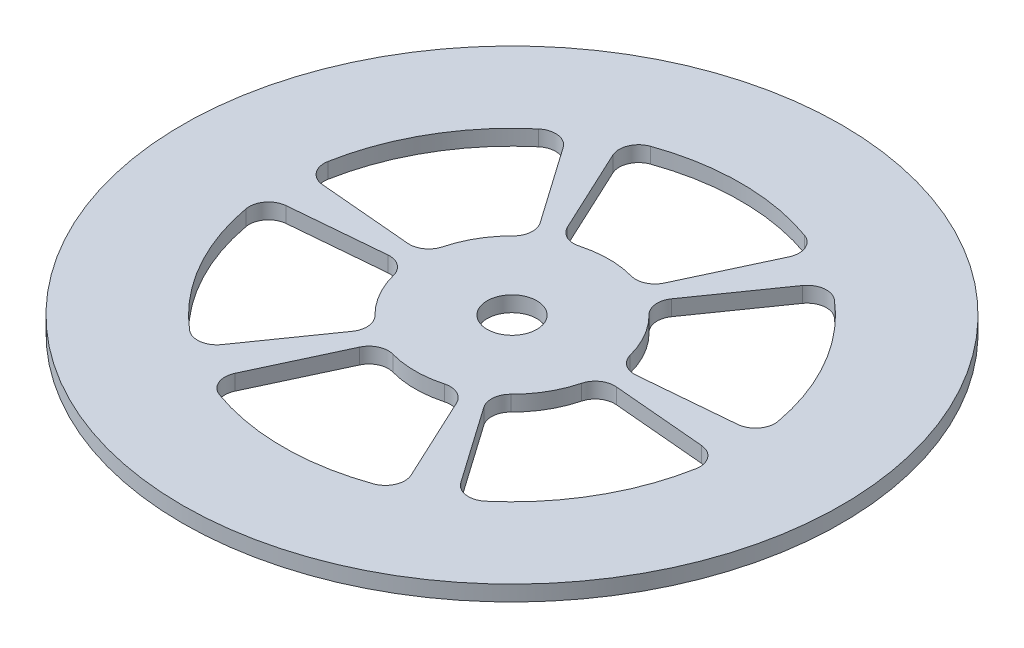
from build123d import *

# Parameters (mm, degrees)
SKETCH1_R           = 85
SKETCH1_R_2         = 6.4
BOSS_EXTRUDE1_DEPTH = 4
CUT_EXTRUDE1_DEPTH  = 10
FILLET1_R           = 5


with BuildPart() as part:
    # Sketch1 → Boss-Extrude1 (new body)
    with BuildSketch(Plane(origin=(0, 0, 0), x_dir=(1, 0, 0), z_dir=(0, 1, 0))):
        with Locations(Location((0, 0, 0), (0, 0, 270))):
            Circle(SKETCH1_R)
        with Locations(Location((0, 0, 0), (0, 0, 270))):
            Circle(SKETCH1_R_2, mode=Mode.SUBTRACT)
    extrude(amount=BOSS_EXTRUDE1_DEPTH)

    # Sketch2 → Cut-Extrude1 (cut)
    with BuildSketch(Plane(origin=(0, 4, 0), x_dir=(1, 0, 0), z_dir=(0, 1, 0))):
        with BuildLine():
            Line((10.565456544, 22.657694676), (24.934477443, 53.472159435))
            ThreePointArc((24.934477443, 53.472159435), (0, 59), (-24.934477443, 53.472159435))
            Line((-24.934477443, 53.472159435), (-10.565456544, 22.657694676))
            ThreePointArc((-10.565456544, 22.657694676), (0, 25), (10.565456544, 22.657694676))
        make_face()
        with BuildLine():
            Line((14.339410909, 20.478801107), (33.841009745, 48.329970613))
            ThreePointArc((33.841009745, 48.329970613), (51.095498823, 29.5), (58.775487187, 5.142188822))
            Line((58.775487187, 5.142188822), (24.904867452, 2.178893569))
            ThreePointArc((24.904867452, 2.178893569), (21.650635095, 12.5), (14.339410909, 20.478801107))
        make_face()
        with BuildLine():
            Line((24.904867452, -2.178893569), (58.775487187, -5.142188822))
            ThreePointArc((58.775487187, -5.142188822), (51.095498823, -29.5), (33.841009745, -48.329970613))
            Line((33.841009745, -48.329970613), (14.339410909, -20.478801107))
            ThreePointArc((14.339410909, -20.478801107), (21.650635095, -12.5), (24.904867452, -2.178893569))
        make_face()
        with BuildLine():
            Line((10.565456544, -22.657694676), (24.934477443, -53.472159435))
            ThreePointArc((24.934477443, -53.472159435), (0, -59), (-24.934477443, -53.472159435))
            Line((-24.934477443, -53.472159435), (-10.565456544, -22.657694676))
            ThreePointArc((-10.565456544, -22.657694676), (0, -25), (10.565456544, -22.657694676))
        make_face()
        with BuildLine():
            Line((-14.339410909, -20.478801107), (-33.841009745, -48.329970613))
            ThreePointArc((-33.841009745, -48.329970613), (-51.095498823, -29.5), (-58.775487187, -5.142188822))
            Line((-58.775487187, -5.142188822), (-24.904867452, -2.178893569))
            ThreePointArc((-24.904867452, -2.178893569), (-21.650635095, -12.5), (-14.339410909, -20.478801107))
        make_face()
        with BuildLine():
            Line((-24.904867452, 2.178893569), (-58.775487187, 5.142188822))
            ThreePointArc((-58.775487187, 5.142188822), (-51.095498823, 29.5), (-33.841009745, 48.329970613))
            Line((-33.841009745, 48.329970613), (-14.339410909, 20.478801107))
            ThreePointArc((-14.339410909, 20.478801107), (-21.650635095, 12.5), (-24.904867452, 2.178893569))
        make_face()
    extrude(amount=-CUT_EXTRUDE1_DEPTH, mode=Mode.SUBTRACT)

    # Fillet1
    fillet1_edges = [part.edges().sort_by_distance(p)[0] for p in [
        (-10.565456544, 2, 22.657694676),
        (10.565456544, 2, 22.657694676),
        (24.934477443, 2, 53.472159435),
        (-24.934477443, 2, 53.472159435),
        (-24.904867452, 2, 2.178893569),
        (-14.339410909, 2, 20.478801107),
        (-33.841009745, 2, 48.329970613),
        (-58.775487187, 2, 5.142188822),
        (14.339410909, 2, 20.478801107),
        (24.904867452, 2, 2.178893569),
        (58.775487187, 2, 5.142188822),
        (33.841009745, 2, 48.329970613),
        (24.904867452, 2, -2.178893569),
        (14.339410909, 2, -20.478801107),
        (33.841009745, 2, -48.329970613),
        (58.775487187, 2, -5.142188822),
        (-14.339410909, 2, -20.478801107),
        (-24.904867452, 2, -2.178893569),
        (-58.775487187, 2, -5.142188822),
        (-33.841009745, 2, -48.329970613),
        (10.565456544, 2, -22.657694676),
        (-10.565456544, 2, -22.657694676),
        (-24.934477443, 2, -53.472159435),
        (24.934477443, 2, -53.472159435),
    ]]
    fillet(fillet1_edges, radius=FILLET1_R)


solid = part.part
